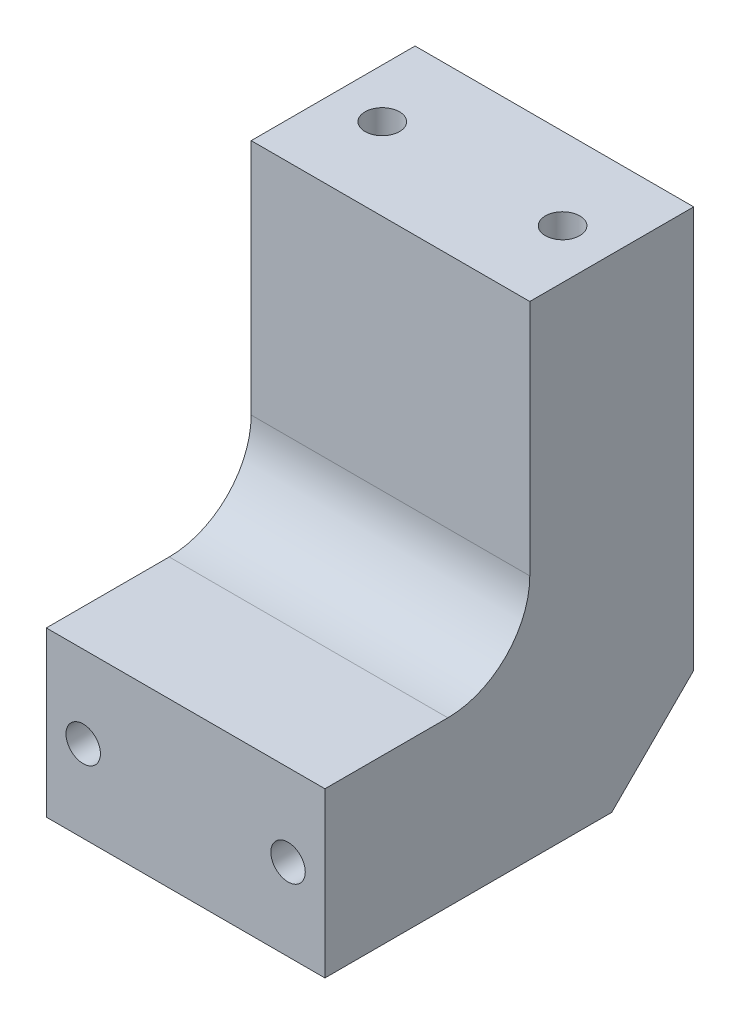
SolidWorks part; units mm, degrees
ref_plane "Front Plane" through (0, 0, 0) normal (0, 0, 1) x (1, 0, 0)
ref_plane "Top Plane" through (0, 0, 0) normal (0, 1, 0) x (1, 0, 0)
ref_plane "Right Plane" through (0, 0, 0) normal (1, 0, 0) x (0, 0, -1)
sketch "Sketch1" plane through (0, 0, 0) normal (0, 1, 0) x (1, 0, 0)
  line L1 (-17, 22.5) -> (17, 22.5)
  line L2 (-17, 22.5) -> (-17, -22.5)
  line L3 (-17, -22.5) -> (17, -22.5)
  line L4 (17, 22.5) -> (17, -22.5)
  line L5 (-17, 22.5) -> (17, -22.5) construction
  line L6 (-17, -22.5) -> (17, 22.5) construction
  point P0 (0, 0)
  dimension "D1" = 34
  dimension "D2" = 45
extrude "Boss-Extrude1" add sketch "Sketch1" along normal blind 59
sketch "Sketch2" plane through (17, 0, 0) normal (1, 0, 0) x (0, 0, -1)
  line L0 (22.5, 59) -> (22.5, 0) construction
  line L1 (-22.5, 59) -> (2.5, 59)
  line L2 (-22.5, 59) -> (-22.5, 20)
  line L3 (-22.5, 20) -> (2.5, 20)
  line L4 (2.5, 59) -> (2.5, 20)
  line L5 (-22.5, 0) -> (22.5, 0) construction
  dimension "D1" = 20
  dimension "D2" = 20
extrude "Cut-Extrude1" cut sketch "Sketch2" against normal blind 45
chamfer "Chamfer1" distance 10 angle 45 1 edges at (0, 0, -22.5)
fillet "Fillet1" radius 10 1 edges at (0, 20, -2.5)
sketch "Sketch4" plane through (0, 59, 0) normal (0, 1, 0) x (1, 0, 0)
  line L0 (0, 0) -> (0, 50000) construction
  line L1 (-20, 12.5) -> (49980, 12.5) construction
  line L2 (-17, 22.5) -> (-17, 2.5) construction
  point P7 (-17, 12.5)
  point P8 (-11, 12.5)
  point P9 (11, 12.5)
  dimension "D1" = 22
hole_wizard "M5 Tapped Hole1" positions "3DSketch1" profile "Sketch5" tap size "M5" standard "Gb"
sketch3d "3DSketch1"
  point P0 (-11, 59, -12.5)
  point P3 (11, 59, -12.5)
sketch "Sketch5" plane through (-11, 59, -12.5) normal (1, 0, 0) x (0, 0, 1)
  line L0 (0, 0) -> (0, 13.6618)
  line L1 (0, 13.6618) -> (2.1, 12.4)
  line L2 (2.1, 12.4) -> (2.1, 0)
  line L5 (2.1, 0) -> (0, 0)
  line L10 (0, 13.6618) -> (-2.1, 12.4) construction
  line L11 (0, -6.35) -> (0, 107.95) construction
  dimension "螺纹孔钻头直径" = 4.2
  dimension "螺纹孔钻头深度" = 12.4
  dimension "导头角度" = 118
cosmetic thread "Cosmetic Thread1" parameters "D1"=10, "D2"=5
cosmetic thread "Cosmetic Thread2" parameters "D1"=10, "D2"=5
sketch "Sketch6" plane through (0, 0, 22.5) normal (0, 0, 1) x (1, 0, 0)
  line L0 (0, 48) -> (0, -49952) construction
  line L1 (17, 59) -> (-17, 59) construction
  line L2 (20, 10) -> (-49980, 10) construction
  line L3 (17, 20) -> (17, 0) construction
  point P4 (0, 59)
  point P9 (17, 10)
  point P10 (-12.5, 10)
  point P11 (12.5, 10)
  dimension "D1" = 25
hole_wizard "M5 Tapped Hole2" positions "3DSketch2" profile "Sketch7" tap size "M5" standard "Gb"
sketch3d "3DSketch2"
  point P0 (-12.5, 10, 22.5)
  point P3 (12.5, 10, 22.5)
sketch "Sketch7" plane through (-12.5, 10, 22.5) normal (1, 0, 0) x (0, -1, 0)
  line L0 (0, 0) -> (0, 13.6618)
  line L1 (0, 13.6618) -> (2.1, 12.4)
  line L2 (2.1, 12.4) -> (2.1, 0)
  line L5 (2.1, 0) -> (0, 0)
  line L10 (0, 13.6618) -> (-2.1, 12.4) construction
  line L11 (0, -6.35) -> (0, 107.95) construction
  dimension "螺纹孔钻头直径" = 4.2
  dimension "螺纹孔钻头深度" = 12.4
  dimension "导头角度" = 118
cosmetic thread "Cosmetic Thread3" parameters "D1"=10, "D2"=5
cosmetic thread "Cosmetic Thread4" parameters "D1"=10, "D2"=5
